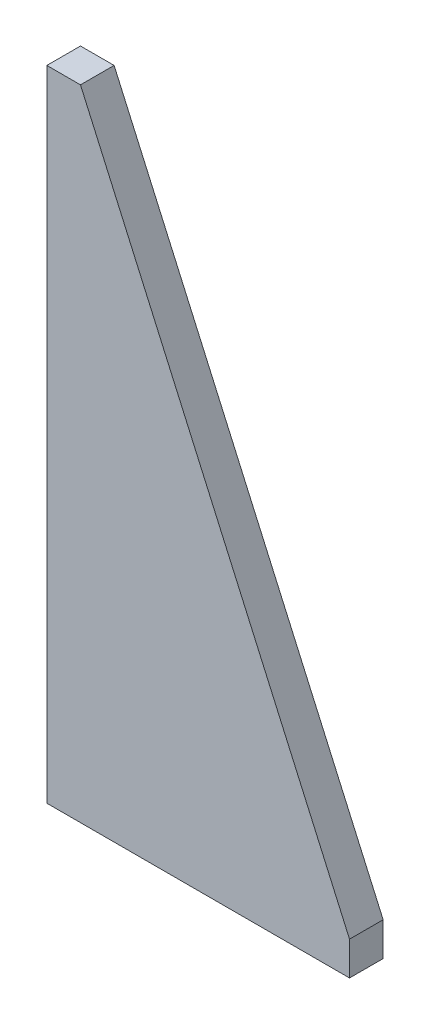
SolidWorks part; units mm, degrees
material "Q235B"
ref_plane "Front Plane" through (0, 0, 0) normal (0, 0, 1) x (1, 0, 0)
ref_plane "Top Plane" through (0, 0, 0) normal (0, 1, 0) x (1, 0, 0)
ref_plane "Right Plane" through (0, 0, 0) normal (1, 0, 0) x (0, 0, -1)
sketch "Sketch1" plane through (0, 0, 0) normal (0, 0, 1) x (1, 0, 0)
  line L0 (0, 0) -> (90, 0)
  line L1 (90, 0) -> (90, 10)
  line L2 (90, 10) -> (10, 190)
  line L3 (10, 190) -> (0, 190)
  line L4 (0, 190) -> (0, 0)
  dimension "D1" = 190
  dimension "D2" = 90
  dimension "D3" = 10
  dimension "D4" = 10
extrude "Boss-Extrude1" add sketch "Sketch1" along normal blind 10
